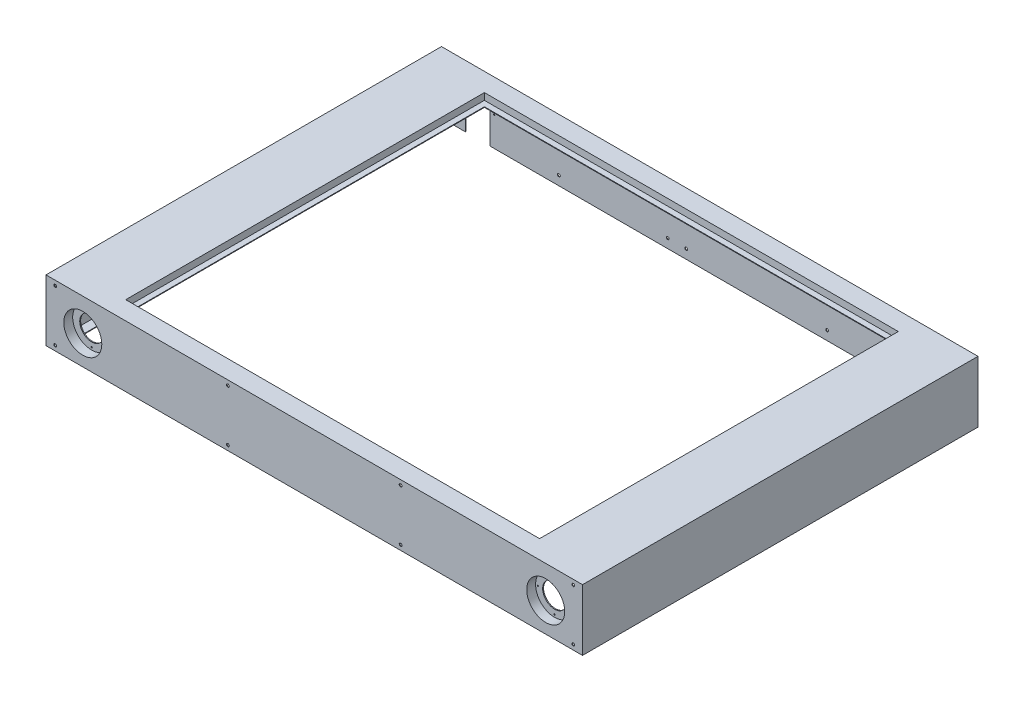
SolidWorks part; units mm, degrees
ref_plane "前视" through (0, 0, 0) normal (0, 0, 1) x (1, 0, 0)
ref_plane "上视" through (0, 0, 0) normal (0, 1, 0) x (1, 0, 0)
ref_plane "右视" through (0, 0, 0) normal (1, 0, 0) x (0, 0, -1)
sketch "草图1" plane through (0, 0, 0) normal (0, 1, 0) x (1, 0, 0)
  line L0 (0, 0) -> (0, 71.9259) construction
  line L1 (0, 0) -> (0, -67.2351) construction
  line L2 (101.6344, 0) -> (-124.4631, 0) construction
  line L4 (-875, 645) -> (875, 645)
  line L5 (-875, 645) -> (-875, -645)
  line L6 (-875, -645) -> (875, -645)
  line L7 (875, 645) -> (875, -645)
  dimension "D1" = 645
  dimension "D2" = 875
  dimension "D3" = 1750
  dimension "D4" = 1290
extrude "凸台-拉伸1" add sketch "草图1" against normal blind 2
sketch "草图2" plane through (0, 0, 0) normal (0, 1, 0) x (-1, 0, 0)
  line L0 (0, 0) -> (0, -429.6525) construction
  line L1 (0, 0) -> (339.6637, 0) construction
  line L2 (-875, -645) -> (875, -645) construction
  line L3 (675, -585) -> (-675, -585)
  line L4 (675, -585) -> (675, 585)
  line L5 (675, 585) -> (-675, 585)
  line L6 (-675, -585) -> (-675, 585)
  line L7 (-875, 645) -> (-875, -645) construction
  dimension "D1" = 60
  dimension "D2" = 200
  dimension "D3" = 1350
  dimension "D4" = 1170
extrude "切除-拉伸1" cut sketch "草图2" against normal blind 2
sketch "草图3" plane through (875, 0, 0) normal (1, 0, 0) x (0, 0, -1)
  line L0 (-645, 0) -> (-645, -200)
  line L1 (-645, 0) -> (645, 0)
  line L2 (645, 0) -> (645, -200)
  line L3 (645, -200) -> (-645, -200)
extrude "凸台-拉伸2" add sketch "草图3" against normal blind 2
sketch "草图4" plane through (0, 0, -645) normal (0, 0, -1) x (-1, 0, 0)
  line L0 (-875, -200) -> (-875, 0)
  line L1 (-875, 0) -> (875, 0)
  line L2 (875, 0) -> (875, -200)
  line L3 (875, -200) -> (-875, -200)
extrude "凸台-拉伸3" add sketch "草图4" against normal blind 2
sketch "草图5" plane through (0, 0, 645) normal (0, 0, 1) x (1, 0, 0)
  line L0 (875, -200) -> (875, 0)
  line L1 (875, 0) -> (-875, 0)
  line L2 (-875, 0) -> (-875, -200)
  line L3 (-875, -200) -> (875, -200)
extrude "凸台-拉伸4" add sketch "草图5" against normal blind 2
sketch "草图6" plane through (-875, 0, 0) normal (-1, 0, 0) x (0, 0, 1)
  line L0 (-645, -200) -> (-645, 0)
  line L1 (-645, 0) -> (645, 0)
  line L2 (645, 0) -> (645, -200)
  line L3 (-645, -200) -> (645, -200)
extrude "凸台-拉伸5" add sketch "草图6" against normal blind 2
sketch "草图7" plane through (0, 0, 0) normal (0, 1, 0) x (1, 0, 0)
  line L0 (-675, 585) -> (-675, -585)
  line L1 (-675, -585) -> (675, -585)
  line L2 (675, -585) -> (675, 585)
  line L3 (675, 585) -> (-675, 585)
  line L5 (-677, 0) -> (-677, 587)
  line L6 (-677, 0) -> (-677, -587)
  line L10 (5, -587) -> (-677, -587)
  line L11 (5, -587) -> (677, -587)
  line L12 (677, 0) -> (677, -587)
  line L13 (677, 0) -> (677, 587)
  line L14 (5, 587) -> (-677, 587)
  line L15 (5, 587) -> (677, 587)
  dimension "D1" = 2
  dimension "D2" = 2
  dimension "D3" = 2
  dimension "D4" = 2
extrude "凸台-拉伸6" add sketch "草图7" against normal blind 24
sketch "草图8" plane through (0, -24, 0) normal (0, -1, 0) x (1, 0, 0)
  line L0 (-677, 587) -> (677, 587)
  line L1 (677, 587) -> (677, -587)
  line L2 (-677, -587) -> (-677, 587)
  line L3 (0, 0) -> (0, 839.0361) construction
  line L4 (0, 0) -> (1020.6379, 0) construction
  line L6 (-657, 567) -> (657, 567)
  line L7 (-657, 567) -> (-657, -567)
  line L8 (-657, -567) -> (657, -567)
  line L9 (657, 567) -> (657, -567)
  line L10 (-677, -587) -> (677, -587)
  dimension "D1" = 20
  dimension "D2" = 20
  dimension "D3" = 20
  dimension "D4" = 20
extrude "凸台-拉伸7" add sketch "草图8" against normal blind 2
sketch "草图9" plane through (0, -200, 0) normal (0, -1, 0) x (1, 0, 0)
  line L0 (-875, 645) -> (875, 645)
  line L1 (875, 645) -> (875, -645)
  line L2 (-845, -610) -> (-845, -645)
  line L3 (-875, -645) -> (-875, 645)
  line L4 (0, 0) -> (0, 373.6588) construction
  line L5 (-845, 615) -> (845, 615)
  line L6 (-845, 615) -> (-845, -610)
  line L7 (-875, -645) -> (875, -645) construction
  line L8 (845, 615) -> (845, -645)
  line L9 (0, 0) -> (328.6397, 0) construction
  line L10 (-845, -645) -> (-875, -645)
  line L12 (845, -645) -> (875, -645)
  dimension "D1" = 30
  dimension "D2" = 30
  dimension "D3" = 30
extrude "凸台-拉伸8" add sketch "草图9" against normal blind 2
sketch "草图10" plane through (0, 0, -645) normal (0, 0, -1) x (-1, 0, 0)
  line L0 (-795, -200) -> (-795, -105)
  line L1 (875, -200) -> (-875, -200) construction
  line L2 (-875, -200) -> (-875, 0) construction
  line L3 (-715, -105) -> (-715, -200)
  line L4 (-795, -200) -> (-715, -200)
  line L5 (715, -200) -> (715, -105)
  line L6 (795, -105) -> (795, -200)
  line L7 (715, -200) -> (795, -200)
  line L8 (875, -200) -> (875, 0) construction
  line L9 (-755, -200) -> (-755, 50.5257) construction
  line L10 (755, -200) -> (755, 27.9332) construction
  arc A0 (-715, -105) -> (-795, -105) centre (-755, -105) ccw
  arc A1 (795, -105) -> (715, -105) centre (755, -105) ccw
  dimension "D3" = 40
  dimension "D4" = 40
  dimension "D7" = 80
  dimension "D1" = 80
  dimension "D2" = 80
  dimension "D5" = 95
  dimension "D6" = 80
  dimension "D8" = 95
extrude "切除-拉伸2" cut sketch "草图10" against normal blind 2
sketch "草图11" plane through (0, 0, -643) normal (0, 0, 1) x (1, 0, 0)
  line L0 (845, 90.2483) -> (845, -355.1183) construction
  line L1 (873, -198) -> (873, -2) construction
  line L2 (875, -200) -> (875, 0) construction
  line L3 (875, 0) -> (-875, 0) construction
  line L4 (795, -200) -> (875, -200) construction
  circle A0 centre (845, -30) radius 4.5
  circle A1 centre (845, -170) radius 4.5
  circle A2 centre (385, -30) radius 4.5
  circle A3 centre (385, -170) radius 4.5
  circle A4 centre (-75, -30) radius 4.5
  circle A5 centre (-75, -170) radius 4.5
  dimension "D2" = 9
  dimension "D3" = 9
  dimension "D4" = 30
  dimension "D5" = 30
  dimension "D1" = 30
  dimension "D6" = 3
extrude "切除-拉伸3" cut sketch "草图11" against normal blind 10
sketch "草图12" plane through (0, 0, -645) normal (0, 0, -1) x (-1, 0, 0)
  line L0 (75, -30) -> (845, -30) construction
  line L1 (845, -30) -> (845, -170) construction
  line L2 (75, -170) -> (845, -170) construction
  line L3 (875, -200) -> (875, 0) construction
  circle A0 centre (845, -30) radius 4.5
  circle A1 centre (845, -170) radius 4.5
  circle A2 centre (490, -30) radius 4.5
  circle A3 centre (490, -170) radius 4.5
  circle A4 centre (135, -30) radius 4.5
  circle A5 centre (135, -170) radius 4.5
  dimension "D2" = 9
  dimension "D3" = 9
  dimension "D1" = 30
  dimension "D5" = 355
  dimension "D4" = 3
extrude "切除-拉伸4" cut sketch "草图12" against normal blind 10
sketch "草图13" plane through (0, -200, 0) normal (0, -1, 0) x (1, 0, 0)
  line L2 (-875, 615) -> (875, 615)
  line L3 (-875, 615) -> (875, 615) construction
  line L11 (-859, -643) -> (-859, 615)
  line L12 (-859, -643) -> (-859, 615) construction
  line L13 (-875, -645) -> (-795, -645) construction
  line L14 (859, 615) -> (859, -643)
  line L15 (859, 615) -> (859, -643) construction
  line L16 (0, 645) -> (0, -752.7243) construction
  line L17 (-875, 645) -> (875, 645) construction
  circle A0 centre (-859, 615) radius 4.5
  circle A1 centre (-859, -615) radius 4.5
  circle A2 centre (859, -615) radius 4.5
  circle A3 centre (859, 615) radius 4.5
  circle A4 centre (859, 320) radius 4.5
  circle A5 centre (859, -150) radius 4.5
  circle A6 centre (-859, 302) radius 4.5
  circle A7 centre (-859, -156.5) radius 4.5
  circle A8 centre (-859, 362) radius 4.5
  circle A9 centre (859, 380) radius 4.5
  dimension "D4" = 30
  dimension "D5" = 9
  dimension "D6" = 9
  dimension "D7" = 9
  dimension "D8" = 9
  dimension "D9" = 295
  dimension "D10" = 470
  dimension "D11" = 9
  dimension "D12" = 917
  dimension "D13" = 9
  dimension "D14" = 458.5
  dimension "D15" = 9
  dimension "D17" = 9
  dimension "D18" = 60
  dimension "D3" = 14
  dimension "D16" = 60
  dimension "D1" = 30
  dimension "D2" = 14
extrude "切除-拉伸5" cut sketch "草图13" against normal blind 10
sketch "草图14" plane through (0, 0, 645) normal (0, 0, 1) x (1, 0, 0)
  line L2 (-845, -200) -> (-845, 0)
  line L3 (-845, -184) -> (-845, -16) construction
  line L5 (845, -200) -> (845, 0)
  line L6 (845, -184) -> (845, -16) construction
  line L8 (-875, -16) -> (875, -16)
  line L9 (-845, -16) -> (845, -16) construction
  line L11 (-875, -184) -> (875, -184)
  line L12 (-845, -184) -> (845, -184) construction
  circle A0 centre (-845, -16) radius 4.5
  circle A1 centre (-281.6667, -16) radius 4.5
  circle A2 centre (281.6667, -16) radius 4.5
  circle A3 centre (845, -16) radius 4.5
  circle A4 centre (-845, -184) radius 4.5
  circle A5 centre (-281.6667, -184) radius 4.5
  circle A6 centre (281.6667, -184) radius 4.5
  circle A7 centre (845, -184) radius 4.5
  dimension "D5" = 9
  dimension "D8" = 563.3333
  dimension "D9" = 563.3333
  dimension "D1" = 30
  dimension "D2" = 30
  dimension "D3" = 16
  dimension "D4" = 16
  dimension "D6" = 4
  dimension "D7" = 2
extrude "切除-拉伸6" cut sketch "草图14" against normal blind 8
sketch "草图16" plane through (0, 0, 645) normal (0, 0, 1) x (1, 0, 0)
  line L0 (-925.3615, -105) -> (1047.9929, -105) construction
  line L1 (-875, -200) -> (-875, 0) construction
  line L2 (-875, 0) -> (875, 0) construction
  line L3 (875, -200) -> (875, 0) construction
  circle A0 centre (755, -105) radius 62
  circle A1 centre (-755, -105) radius 62
  dimension "D1" = 120
  dimension "D3" = 120
  dimension "D4" = 124
  dimension "D5" = 124
  dimension "D2" = 105
extrude "切除-拉伸7" cut sketch "草图16" against normal blind 10
sketch "草图17" plane through (0, 0, 643) normal (0, 0, -1) x (-1, 0, 0)
  circle A3 centre (-755, -105) radius 64
  circle A4 centre (-755, -105) radius 62
  dimension "D1" = 2
extrude "凸台-拉伸9" add sketch "草图17" along normal blind 27
ref_plane "基准面1" through (0, 0, 0) normal (-1, 0, 0) x (0, 0, 1)
sketch "草图22" plane through (0, 0, 616) normal (0, 0, -1) x (-1, 0, 0)
  circle A0 centre (-755, -105) radius 64
  circle A1 centre (-755, -105) radius 39
  circle A2 centre (-755, -105) radius 64 construction
  dimension "D1" = 78
extrude "凸台-拉伸11" add sketch "草图22" along normal blind 3
mirror "镜向2" about plane through (0, 0, 0) normal (-1, 0, 0) of "凸台-拉伸11", "凸台-拉伸9"
hole_wizard "M5 螺纹孔1" positions "草图24" profile "草图23" tap size "M5" standard "GB"
sketch "草图24" plane through (0, 0, 616) normal (0, 0, 1) x (1, 0, 0)
  line L0 (755, -105) -> (755, -28.6713) construction
  line L2 (755, -105) -> (707.4596, -22.6577) construction
  line L4 (755, -105) -> (658.8381, -105) construction
  line L6 (755, -105) -> (755, -186.1629) construction
  line L8 (755, -159) -> (914.4585, -159) construction
  circle A0 centre (755, -105) radius 54 construction
  point P0 (728, -58.2346)
  point P1 (701, -105)
  point P3 (755, -159)
  point P40 (800, -159)
  dimension "D1" = 108
  dimension "D2" = 30
  dimension "D3" = 45
sketch "草图23" plane through (728, -58.2346, 616) normal (1, 0, 0) x (0, -1, 0)
  line L0 (0, 0) -> (0, 1261)
  line L1 (0, 1261) -> (2.1, 1261)
  line L2 (2.1, 1261) -> (2.1, 0)
  line L5 (2.1, 0) -> (0, 0)
  line L11 (0, -6.35) -> (0, 107.95) construction
  dimension "通孔螺纹孔钻头直径" = 4.2
  dimension "通孔螺纹孔钻头深度" = 1261
cosmetic thread "孔螺蚊线1" parameters "D2"=5
cosmetic thread "孔螺蚊线2" parameters "D2"=5
cosmetic thread "孔螺蚊线3" parameters "D2"=5
cosmetic thread "孔螺蚊线4" parameters "D2"=5
mirror "镜向3" about plane through (0, 0, 0) normal (-1, 0, 0) of "M5 螺纹孔1"
